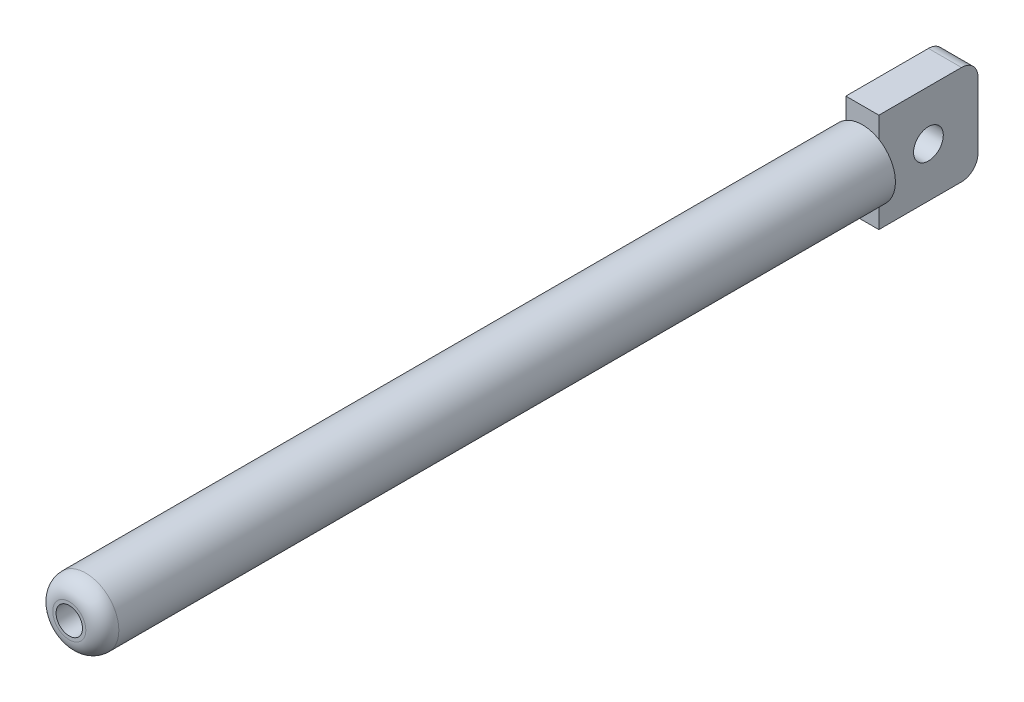
SolidWorks part; units mm, degrees
ref_plane "Front Plane" through (0, 0, 0) normal (0, 0, 1) x (1, 0, 0)
ref_plane "Top Plane" through (0, 0, 0) normal (0, 1, 0) x (1, 0, 0)
ref_plane "Right Plane" through (0, 0, 0) normal (1, 0, 0) x (0, 0, -1)
sketch "Sketch1" plane through (0, 0, 0) normal (0, 0, 1) x (1, 0, 0)
  circle A0 centre (0, 0) radius 10
  dimension "D1" = 20
extrude "Boss-Extrude1" add sketch "Sketch1" along normal blind 240
sketch "Sketch2" plane through (0, 0, 0) normal (1, 0, 0) x (0, 0, -1)
  line L0 (0, 0) -> (39.0993, 0) construction
  line L1 (11, 0) -> (-11, 0) construction
  line L2 (0, -15) -> (0, 15)
  line L3 (0, 15) -> (30, 15)
  line L4 (30, -15) -> (30, 15)
  line L5 (0, -15) -> (30, -15)
  point P9 (30, 0)
  dimension "D1" = 30
  dimension "D2" = 15
extrude "Boss-Extrude2" add sketch "Sketch2" along normal mid plane 10
sketch "Sketch3" plane through (5, 0, 0) normal (1, 0, 0) x (0, 0, -1)
  line L0 (30, -15) -> (30, 15) construction
  circle A0 centre (15, 0) radius 4.5
  dimension "D1" = 9
  dimension "D2" = 15
extrude "Cut-Extrude1" cut sketch "Sketch3" against normal blind 38
fillet "Fillet1" radius 5 2 edges at (0, 15, -30) (0, -15, -30)
fillet "Fillet2" radius 5 1 edges at (10, 0, 240)
sketch "Sketch4" plane through (0, 0, 240) normal (0, 0, 1) x (1, 0, 0)
  circle A0 centre (0, 0) radius 4
  dimension "D1" = 8
extrude "Cut-Extrude2" cut sketch "Sketch4" against normal blind 20
